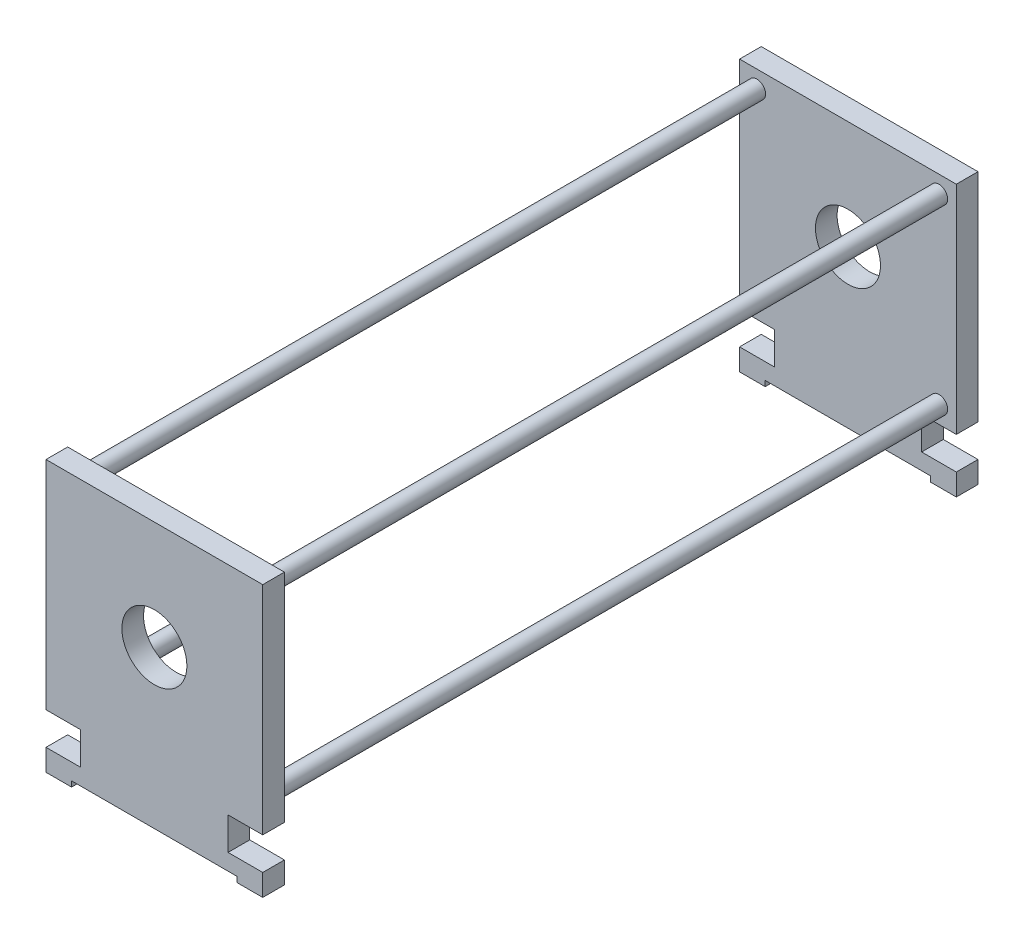
from build123d import *

# Parameters (mm, degrees)
SKETCH1_R           = 30
BOSS_EXTRUDE1_DEPTH = 20
SKETCH2_R           = 8
BOSS_EXTRUDE2_DEPTH = 620
SKETCH3_R           = 30
BOSS_EXTRUDE3_DEPTH = 20


with BuildPart() as part:
    # Sketch1 → Boss-Extrude1 (new body)
    with BuildSketch(Plane.XY):
        Polygon((76.388888889, 0), (-76.388888889, 0), (-76.388888889, -5), (-100, -5), (-100, 15), (-68, 15), (-68, 45), (-100, 45), (-100, 245), (100, 245), (100, 45), (68, 45), (68, 15), (100, 15), (100, -5), (76.388888889, -5), align=None)
        with Locations((0, 145)):
            Circle(SKETCH1_R, mode=Mode.SUBTRACT)
    extrude(amount=BOSS_EXTRUDE1_DEPTH)

    # Sketch2 → Boss-Extrude2 (add)
    with BuildSketch(Plane.XY.offset(20)):
        with Locations(Location((-84, 229, 0), (0, 0, 180))):
            Circle(SKETCH2_R)
        with Locations(Location((84, 229, 0), (0, 0, 180))):
            Circle(SKETCH2_R)
        with Locations(Location((84, 61, 0), (0, 0, 180))):
            Circle(SKETCH2_R)
        with Locations(Location((-84, 61, 0), (0, 0, 180))):
            Circle(SKETCH2_R)
    extrude(amount=BOSS_EXTRUDE2_DEPTH)

    # Sketch3 → Boss-Extrude3 (add)
    with BuildSketch(Plane.XY.offset(640)):
        Polygon((76.388888889, 0), (-76.388888889, 0), (-76.388888889, -5), (-100, -5), (-100, 15), (-68, 15), (-68, 45), (-100, 45), (-100, 245), (100, 245), (100, 45), (68, 45), (68, 15), (100, 15), (100, -5), (76.388888889, -5), align=None)
        with Locations((0, 145)):
            Circle(SKETCH3_R, mode=Mode.SUBTRACT)
    extrude(amount=BOSS_EXTRUDE3_DEPTH)


solid = part.part
